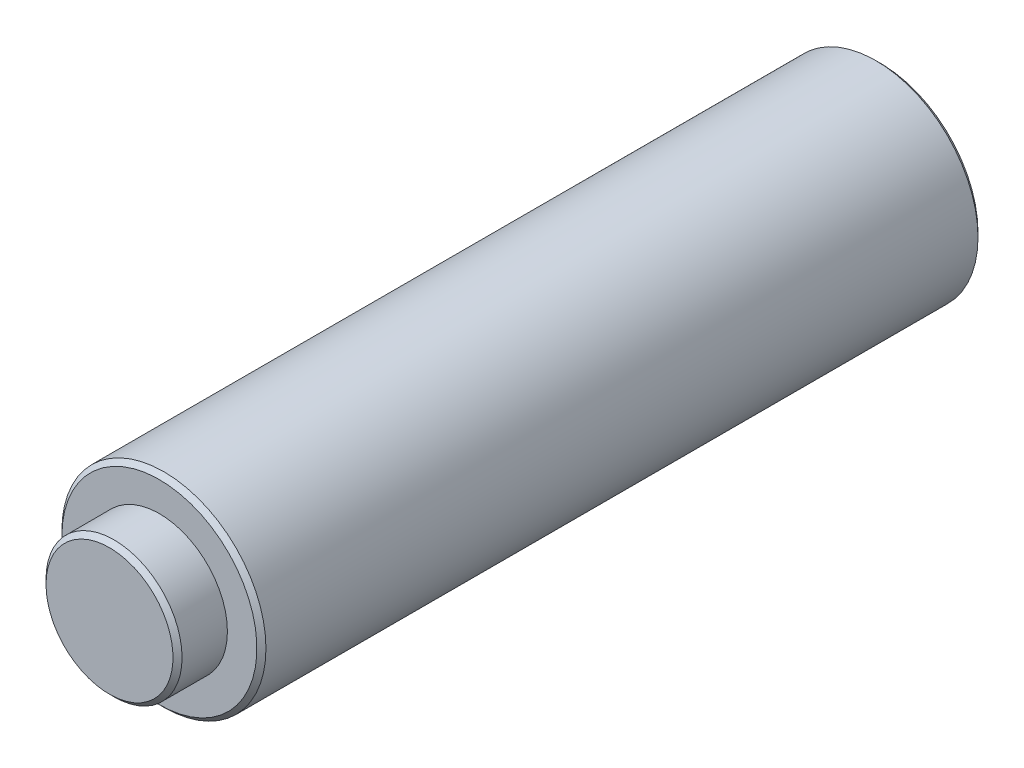
SolidWorks part; units mm, degrees
material "Q235B"
ref_plane "Front Plane" through (0, 0, 0) normal (0, 0, 1) x (1, 0, 0)
ref_plane "Top Plane" through (0, 0, 0) normal (0, 1, 0) x (1, 0, 0)
ref_plane "Right Plane" through (0, 0, 0) normal (1, 0, 0) x (0, 0, -1)
sketch "Sketch1" plane through (0, 0, 0) normal (1, 0, 0) x (0, 0, -1)
  line L0 (0, 0) -> (178, 0) construction
  line L1 (178, 0) -> (178, 9)
  line L2 (178, 9) -> (170, 9)
  line L3 (170, 9) -> (170, 22.5)
  line L4 (170, 22.5) -> (11, 22.5)
  line L5 (11, 22.5) -> (11, 15)
  line L6 (11, 15) -> (0, 15)
  line L7 (0, 15) -> (0, 0)
  line L8 (0, 0) -> (178, 0)
  dimension "D1" = 45
  dimension "D2" = 30
  dimension "D3" = 11
  dimension "D4" = 159
  dimension "D5" = 18
  dimension "D6" = 8
revolve "Revolve1" add sketch "Sketch1" angle 360 about L0
chamfer "Chamfer1" distance 1 angle 45 4 edges at (15, 0, 0) (22.5, 0, -11) (9, 0, -178) (22.5, 0, -170)
